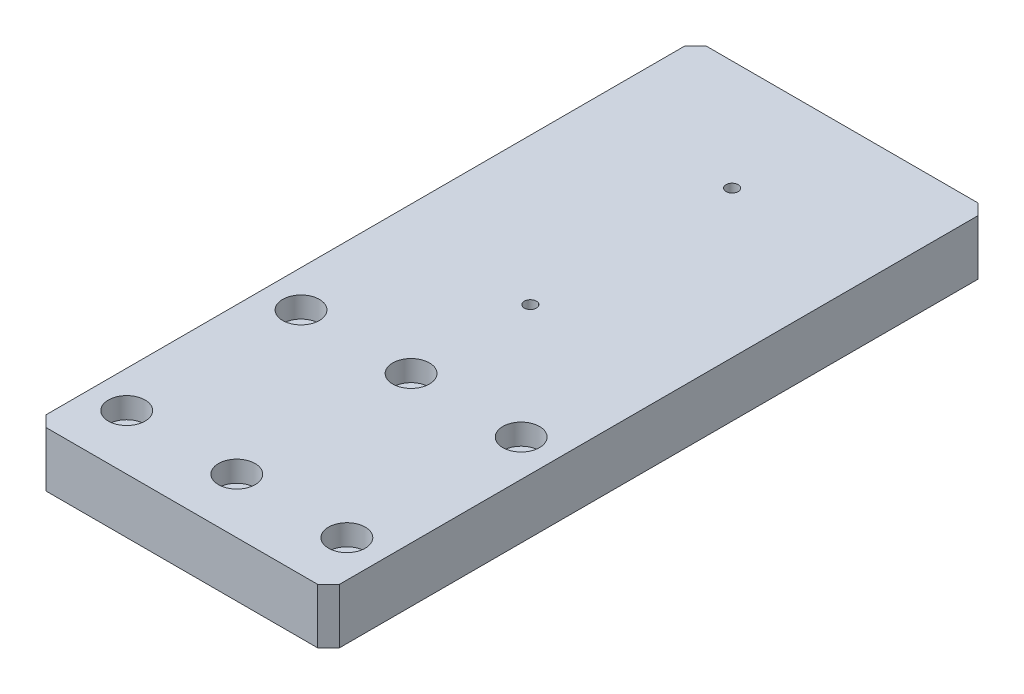
SolidWorks part; units mm, degrees
material "A6061 T6"
ref_plane "前视基准面" through (0, 0, 0) normal (0, 0, 1) x (1, 0, 0)
ref_plane "上视基准面" through (0, 0, 0) normal (0, 1, 0) x (1, 0, 0)
ref_plane "右视基准面" through (0, 0, 0) normal (1, 0, 0) x (0, 0, -1)
sketch "草图1" plane through (0, 0, 0) normal (0, 1, 0) x (1, 0, 0)
  line L1 (-40, 90) -> (40, 90)
  line L2 (-40, 90) -> (-40, -90)
  line L3 (-40, -90) -> (40, -90)
  line L4 (40, 90) -> (40, -90)
  line L5 (-40, 90) -> (40, -90) construction
  line L6 (-40, -90) -> (40, 90) construction
  point P0 (0, 0)
  dimension "D1" = 80
  dimension "D2" = 180
extrude "凸台-拉伸1" add sketch "草图1" along normal blind 15
chamfer "倒角1" distance 3 angle 45 4 edges at (-40, 7.5, -90) (40, 7.5, -90) (40, 7.5, 90) (-40, 7.5, 90)
hole_wizard "M4 螺纹孔1" positions "草图4" profile "草图3" tap size "M4" standard "GB"
sketch "草图4" plane through (0, 15, 0) normal (0, 1, 0) x (1, 0, 0)
  point P0 (0, 60)
  point P3 (0, 5)
sketch "草图3" plane through (0, 15, -60) normal (1, 0, 0) x (0, 0, 1)
  line L0 (0, 0) -> (0, 20.9914)
  line L1 (0, 20.9914) -> (1.65, 20)
  line L2 (1.65, 20) -> (1.65, 0)
  line L5 (1.65, 0) -> (0, 0)
  line L10 (0, 20.9914) -> (-1.65, 20) construction
  line L11 (0, -6.35) -> (0, 107.95) construction
  dimension "螺纹孔钻头直径" = 3.3
  dimension "螺纹孔钻头深度" = 20
  dimension "导头角度" = 118
cosmetic thread "孔螺蚊线1"
cosmetic thread "孔螺蚊线2"
hole_wizard "打孔尺寸(%根据)内六角圆柱头螺钉的类型1" positions "草图5" profile "草图6" counterbore size "M5" standard "GB"
sketch "草图5" plane through (0, 15, 0) normal (0, 1, 0) x (1, 0, 0)
  line L0 (-37, -90) -> (37, -90) construction
  line L1 (-40, 87) -> (-40, -87) construction
  line L2 (40, -87) -> (40, 87) construction
  point P0 (-30, -27.5)
  point P2 (0, -27.5)
  point P4 (30, -27.5)
  dimension "D1" = 62.5
  dimension "D2" = 10
  dimension "D3" = 10
  dimension "D4" = 30
sketch "草图6" plane through (-30, 15, 27.5) normal (1, 0, 0) x (0, 0, 1)
  line L0 (0, 0) -> (0, 21.6524)
  line L1 (0, 21.6524) -> (2.75, 20)
  line L2 (2.75, 20) -> (2.75, 5.7)
  line L3 (2.75, 5.7) -> (5, 5.7)
  line L4 (5, 5.7) -> (5, 0)
  line L5 (5, 0) -> (0, 0)
  line L10 (0, 21.6524) -> (-2.75, 20) construction
  line L11 (0, -6.35) -> (0, 107.95) construction
  dimension "孔直径" = 5.5
  dimension "孔深度" = 20
  dimension "柱形沉头孔直径" = 10
  dimension "柱形沉头孔深度" = 5.7
  dimension "导头角度" = 118
hole_wizard "打孔尺寸(%根据)内六角圆柱头螺钉的类型2" positions "草图7" profile "草图8" counterbore size "M5" standard "GB"
sketch "草图7" plane through (0, 15, 0) normal (0, 1, 0) x (1, 0, 0)
  line L0 (-37, -90) -> (37, -90) construction
  line L1 (-40, 87) -> (-40, -87) construction
  line L2 (40, -87) -> (40, 87) construction
  point P0 (-30, -75)
  point P2 (0, -75)
  point P4 (30, -75)
  dimension "D1" = 15
  dimension "D2" = 10
  dimension "D3" = 10
  dimension "D4" = 30
sketch "草图8" plane through (-30, 15, 75) normal (1, 0, 0) x (0, 0, 1)
  line L0 (0, 0) -> (0, 16.6524)
  line L1 (0, 16.6524) -> (2.75, 15)
  line L2 (2.75, 15) -> (2.75, 5.7)
  line L3 (2.75, 5.7) -> (5, 5.7)
  line L4 (5, 5.7) -> (5, 0)
  line L5 (5, 0) -> (0, 0)
  line L10 (0, 16.6524) -> (-2.75, 15) construction
  line L11 (0, -6.35) -> (0, 107.95) construction
  dimension "孔直径" = 5.5
  dimension "孔深度" = 15
  dimension "柱形沉头孔直径" = 10
  dimension "柱形沉头孔深度" = 5.7
  dimension "导头角度" = 118
